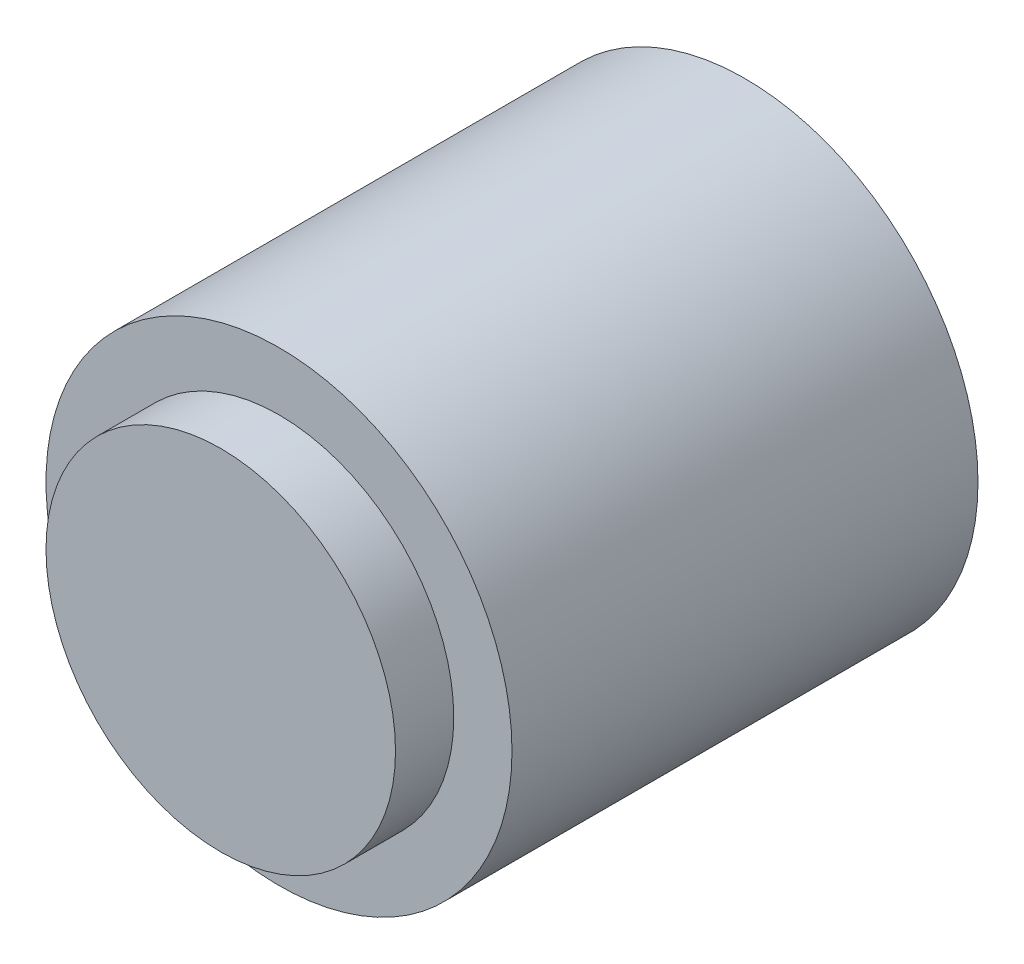
from build123d import *

# Parameters (mm, degrees)
SKETCH1_R           = 20
BOSS_EXTRUDE1_DEPTH = 40
SKETCH2_R           = 15
BOSS_EXTRUDE2_DEPTH = 5


with BuildPart() as part:
    # Sketch1 → Boss-Extrude1 (new body)
    with BuildSketch(Plane.XY):
        Circle(SKETCH1_R)
    extrude(amount=BOSS_EXTRUDE1_DEPTH)

    # Sketch2 → Boss-Extrude2 (add)
    with BuildSketch(Plane.XY.offset(40)):
        Circle(SKETCH2_R)
    extrude(amount=BOSS_EXTRUDE2_DEPTH)


solid = part.part
